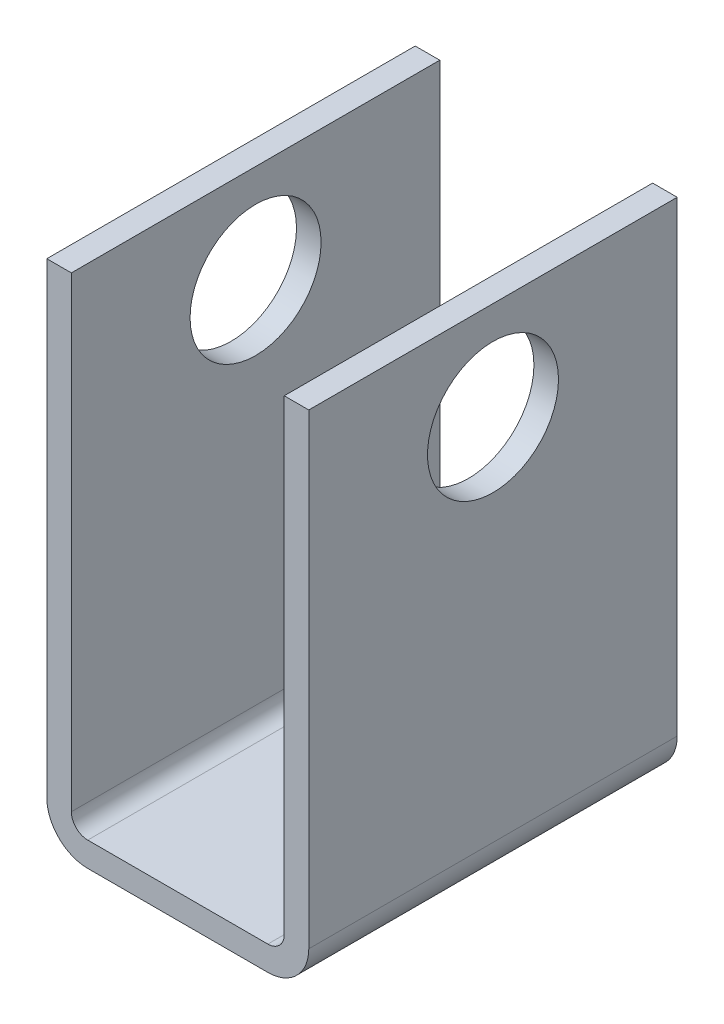
SolidWorks part; units mm, degrees
ref_plane "Front Plane" through (0, 0, 0) normal (0, 0, 1) x (1, 0, 0)
ref_plane "Top Plane" through (0, 0, 0) normal (0, 1, 0) x (1, 0, 0)
ref_plane "Right Plane" through (0, 0, 0) normal (1, 0, 0) x (0, 0, -1)
sketch "Sketch1" plane through (0, 0, 0) normal (0, 0, 1) x (1, 0, 0)
  line L0 (0, 0) -> (0, -57)
  line L1 (5, -62) -> (27, -62)
  line L2 (32, -57) -> (32, 0)
  line L3 (3, 0) -> (3, -57)
  line L4 (5, -59) -> (27, -59)
  line L5 (29, -57) -> (29, 0)
  line L6 (3, 0) -> (0, 0)
  line L7 (29, 0) -> (32, 0)
  arc A0 (27, -62) -> (32, -57) centre (27, -57) ccw
  arc A1 (0, -57) -> (5, -62) centre (5, -57) ccw
  arc A2 (3, -57) -> (5, -59) centre (5, -57) ccw
  arc A3 (27, -59) -> (29, -57) centre (27, -57) ccw
  point P8 (32, -62)
  point P11 (0, -62)
  dimension "D3" = 5
  dimension "D1" = 32
  dimension "D2" = 62
  dimension "D4" = 3
extrude "Boss-Extrude1" add sketch "Sketch1" along normal blind 45
sketch "Sketch2" plane through (32, 0, 0) normal (1, 0, 0) x (0, 0, -1)
  line L0 (0, -57) -> (0, 0) construction
  line L1 (-45, 0) -> (0, 0) construction
  circle A0 centre (-22.5, -12) radius 8
  dimension "D1" = 16
  dimension "D2" = 22.5
  dimension "D3" = 12
extrude "Cut-Extrude1" cut sketch "Sketch2" against normal through all
